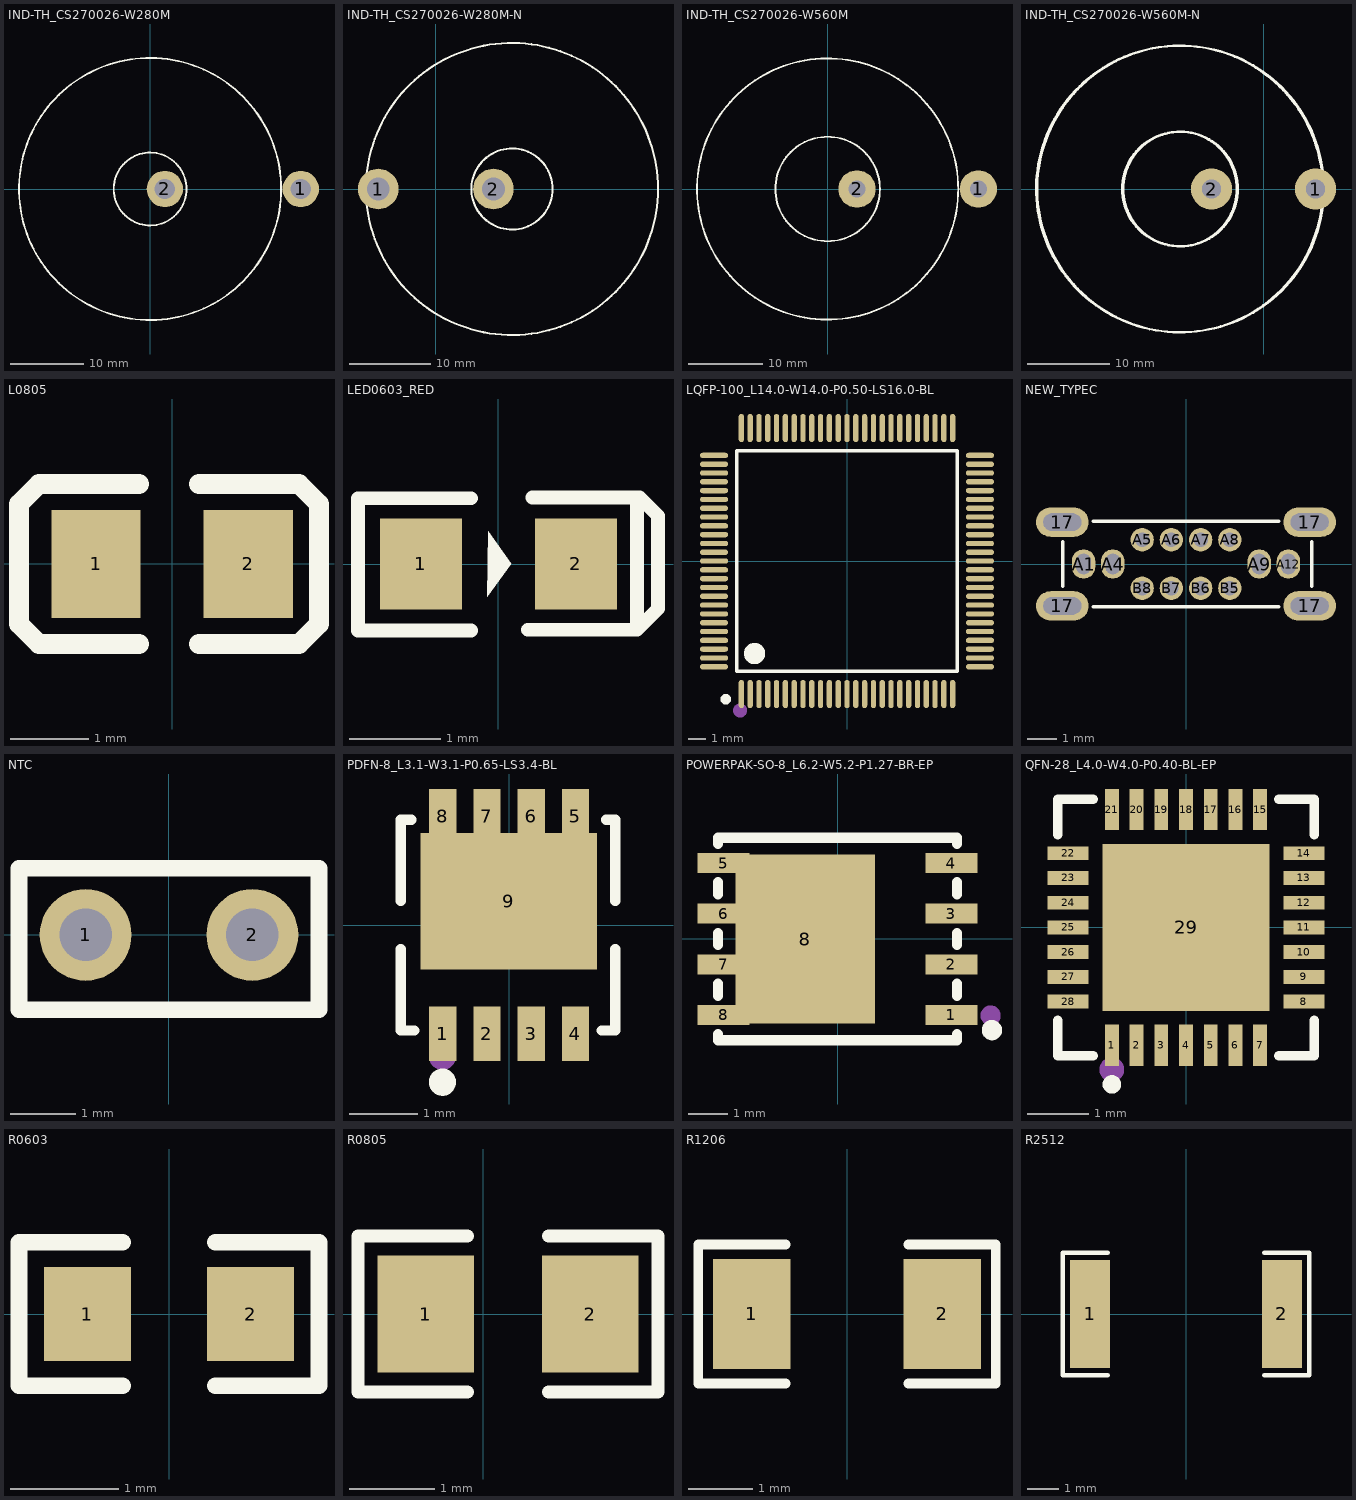
[diagram p0: the footprints below, top view; thin cyan lines are the x and y axes]
# Altium footprint library MISC84402-3.PcbLib: 74 footprints (part 3 of 5)
Each footprint in its own frame and in the unit in brackets; x right, y up, seen from the top. Pads: shape width x height; smd on the part's side, far side on the other; paste and mask are expansions set on the pad; w line width, h text height; cw(c..) or ccw(c..) is an arc to the next point about the centre after c.

## IND-TH_CS270026-W280M [mm]
pads (2):
  round 5 hole 2.8: 1(20.701,0) 2(2.032,0)
Top Overlay:
  circle w0.254: c0,0 r18
  circle w0.254: c0,0 r5

## IND-TH_CS270026-W280M-N [mm]
pads (2):
  round 5 hole 2.8: 1(-7.096,0) 2(7.096,0)
Top Overlay:
  circle w0.254: c7.096,0 r1.4
  circle w0.254: c-7.096,0 r1.4
  circle w0.254: c9.385,0.001 r18
  circle w0.254: c9.385,0 r5
  lines w0.254: 7.096,-1.4 cw(c7.096,0) 7.096,1.4 ; 7.096,-1.4 7.101,-1.4 7.096,-1.4 ; 7.096,1.4 7.101,1.4 7.096,1.4

## IND-TH_CS270026-W560M [mm]
pads (2):
  round 5 hole 2.3: 1(20.193,0) 2(3.937,0)
Top Overlay:
  circle w0.254: c0,0 r7
  circle w0.254: c0,0 r17.5

## IND-TH_CS270026-W560M-N [mm]
pads (2):
  round 5 hole 2.3 slot 2.305 at 0 deg: 1(6.35,0) 2(-6.35,0)
Top Overlay:
  circle w0.254: c6.281,0.04 r1.15
  circle w0.254: c-6.17,-0.013 r1.15
  circle w0.254: c-10.11,-0.013 r7
  circle w0.254: c-10.11,-0.013 r17.5
  circle w0.254: c-10.112,0.013 r17.5
  circle w0.254: c-10.112,0.013 r7
  lines w0.254: -10.287,-17.5 cw(c-10.284,0) -10.281,-17.5 ; -10.287,-7 cw(c-10.288,0) -10.28,-7 ; -6.175,-1.174 -6.17,-1.174 ; -6.175,-1.174 -6.17,-1.174 ; -6.175,-1.174 -6.17,-1.174 ; -6.175,-1.174 -6.17,-1.174 ; -6.175,1.149 -6.17,1.149 ; -6.175,1.149 -6.17,1.149 ; -6.175,1.149 -6.17,1.149 ; -6.175,1.149 -6.17,1.149 ; -6.175,-1.163 -6.17,-1.163 -6.175,-1.163 ; -6.175,1.137 -6.17,1.137 -6.175,1.137

## L0805 [mm]
pads (2):
  rect 1.133x1.377 smd: 1(-0.966,0) 2(0.966,0)
Top Overlay:
  lines w0.254: -0.421,-1.016 -1.691,-1.016 -1.945,-0.762 -1.945,-0.635 -1.945,0.762 -1.691,1.016 -1.564,1.016 -0.421,1.016 ; 0.341,-1.016 1.484,-1.016 1.611,-1.016 1.865,-0.762 1.865,0.635 1.865,0.762 1.611,1.016 0.341,1.016
Top Paste:
  region: 0.36,-0.22 0.36,0.22 0.745,0.688 1.433,0.688 1.533,0.588 1.533,-0.589 1.433,-0.689 0.745,-0.689
  region: -0.36,-0.22 -0.36,0.22 -0.745,0.688 -1.433,0.688 -1.533,0.588 -1.533,-0.589 -1.433,-0.689 -0.745,-0.689

## LED0603_RED [mm]
pads (2):
  rect 0.9x1 smd: 1(-0.85,0) 2(0.85,0)
Top Overlay:
  region: -0.11,0.36 -0.12,-0.36 0.14,0
  lines w0.15: -0.3,-0.73 -1.54,-0.73 -1.54,0.72 -0.3,0.72 ; 0.32,-0.72 1.52,-0.72 ; 0.37,0.73 1.52,0.73 ; 1.52,-0.72 1.72,-0.52 1.75,-0.49 1.75,0.53 1.55,0.73 1.52,0.73 ; 1.52,-0.72 1.52,0.73

## LQFP-100_L14.0-W14.0-P0.50-LS16.0-BL [mm]
pads (100):
  oval 0.3x1.6 smd: 1(-6,-7.55) 2(-5.5,-7.55) 3(-5,-7.55) 4(-4.5,-7.55) 5(-4,-7.55) 6(-3.5,-7.55) 7(-3,-7.55) 8(-2.5,-7.55) 9(-2,-7.55) 10(-1.5,-7.55) 11(-1,-7.55) 12(-0.5,-7.55) 13(0,-7.55) 14(0.5,-7.55) 15(1,-7.55) 16(1.5,-7.55) 17(2,-7.55) 18(2.5,-7.55) 19(3,-7.55) 20(3.5,-7.55) 21(4,-7.55) 22(4.5,-7.55) 23(5,-7.55) 24(5.5,-7.55) 25(6,-7.55) 51(6,7.55) 52(5.5,7.55) 53(5,7.55) 54(4.5,7.55) 55(4,7.55) 56(3.5,7.55) 57(3,7.55) 58(2.5,7.55) 59(2,7.55) 60(1.5,7.55) 61(1,7.55) 62(0.5,7.55) 63(0,7.55) 64(-0.5,7.55) 65(-1,7.55) 66(-1.5,7.55) 67(-2,7.55) 68(-2.5,7.55) 69(-3,7.55) 70(-3.5,7.55) 71(-4,7.55) 72(-4.5,7.55) 73(-5,7.55) 74(-5.5,7.55) 75(-6,7.55)
  oval 1.6x0.3 smd: 26(7.55,-6) 27(7.55,-5.5) 28(7.55,-5) 29(7.55,-4.5) 30(7.55,-4) 31(7.55,-3.5) 32(7.55,-3) 33(7.55,-2.5) 34(7.55,-2) 35(7.55,-1.5) 36(7.55,-1) 37(7.55,-0.5) 38(7.55,0) 39(7.55,0.5) 40(7.55,1) 41(7.55,1.5) 42(7.55,2) 43(7.55,2.5) 44(7.55,3) 45(7.55,3.5) 46(7.55,4) 47(7.55,4.5) 48(7.55,5) 49(7.55,5.5) 50(7.55,6) 76(-7.55,6) 77(-7.55,5.5) 78(-7.55,5) 79(-7.55,4.5) 80(-7.55,4) 81(-7.55,3.5) 82(-7.55,3) 83(-7.55,2.5) 84(-7.55,2) 85(-7.55,1.5) 86(-7.55,1) 87(-7.55,0.5) 88(-7.55,0) 89(-7.55,-0.5) 90(-7.55,-1) 91(-7.55,-1.5) 92(-7.55,-2) 93(-7.55,-2.5) 94(-7.55,-3) 95(-7.55,-3.5) 96(-7.55,-4) 97(-7.55,-4.5) 98(-7.55,-5) 99(-7.55,-5.5) 100(-7.55,-6)
Top Overlay:
  lines w0.2: -6.25,-6.25 6.25,-6.25 6.25,6.25 -6.25,6.25 -6.25,-6.25
  lines w0.3: -6.883,-7.696 ccw(c-6.882,-7.846) -6.881,-7.696
  lines w0.6: -5.25,-4.95 ccw(c-5.248,-5.25) -5.245,-4.95
Mechanical 15:
  circle w0.4: c-6.071,-8.484 r0.2

## NEW_TYPEC [mm]
pads (16):
  oval 1.8x1 hole 0.6 slot 1.3 at 0 deg: 17(-4.225,-1.43) 17(-4.225,1.43) 17(4.225,-1.43) 17(4.225,1.43)
  oval 0.8x1 hole 0.5 slot 0.7 at 90 deg: A1(-3.5,0) A4(-2.5,0) A9(2.5,0) A12(3.5,0)
  round 0.8 hole 0.5: A5(-1.5,0.825) A6(-0.5,0.825) A7(0.5,0.825) A8(1.5,0.825) B5(1.5,-0.825) B6(0.5,-0.825) B7(-0.5,-0.825) B8(-1.5,-0.825)
Top Overlay:
  lines w0.127: -4.215,-0.762 -4.215,0.762 ; -3.158,-1.46 3.158,-1.46 ; -3.158,1.461 3.158,1.461 ; 4.294,-0.762 4.294,0.762

## NTC [mm]
pads (2):
  round 1.4 hole 0.8: 1(-1.27,0) 2(1.27,0)
Top Overlay:
  lines w0.254: -2.286,-1.143 2.286,-1.143 2.286,1.016 -2.286,1.016 -2.286,-1.143

## PDFN-8_L3.1-W3.1-P0.65-LS3.4-BL [mm]
pads (9):
  rect 0.4x0.8 smd: 1(-0.975,-1.6) 2(-0.325,-1.6) 3(0.325,-1.6) 4(0.975,-1.6) 5(0.975,1.6) 6(0.325,1.6) 7(-0.325,1.6) 8(-0.975,1.6)
  rect 2.6x2 smd: 9(-0.005,0.35)
Top Overlay:
  circle w0.2: c-0.98,-2.31 r0.1
  lines w0.152: -1.592,-0.354 -1.592,-1.55 -1.396,-1.55 ; -1.592,0.354 -1.592,1.55 -1.434,1.55 ; 1.362,-1.55 1.56,-1.55 1.56,-0.354 ; 1.425,1.55 1.56,1.55 1.56,0.354
Top Paste:
  region: 1.175,1.5 0.775,1.5 0.775,2 1.175,2
  region: 0.525,1.5 0.125,1.5 0.125,2 0.525,2
  region: -0.125,1.5 -0.525,1.5 -0.525,2 -0.125,2
  region: -1.31,1.22 1.293,1.22 1.293,-0.649 -1.307,-0.649
  region: -1.175,-2 -1.175,-1.2 -0.775,-1.2 -0.775,-2
  region: -0.525,-2 -0.525,-1.2 -0.125,-1.2 -0.125,-2
  region: 0.125,-2 0.125,-1.2 0.525,-1.2 0.525,-2
  region: 0.775,-2 0.775,-1.2 1.175,-1.2 1.175,-2
  region: -0.775,1.5 -1.175,1.5 -1.175,2 -0.775,2
Mechanical 15:
  circle w0.2: c-0.98,-1.93 r0.1

## POWERPAK-SO-8_L6.2-W5.2-P1.27-BR-EP [mm]
pads (9):
  rect 1.3x0.5 smd: 1(2.858,-1.905) 2(2.858,-0.635) 3(2.858,0.635) 4(2.858,1.905) 5(-2.858,1.905) 6(-2.858,0.635) 7(-2.858,-0.635) 8(-2.858,-1.905)
  rect 3.5x4.25 smd: 8(-0.813,0)
Top Overlay:
  circle w0.254: c3.873,-2.286 r0.127
  lines w0.254: -3,-2.386 -3,-2.54 3,-2.54 3,-2.386 ; -3,-1.424 -3,-1.116 ; -3,-0.154 -3,0.154 ; -3,1.116 -3,1.424 ; -3,2.386 -3,2.54 3,2.54 3,2.386 ; 3,-1.424 3,-1.116 ; 3,-0.154 3,0.154 ; 3,1.116 3,1.424
Top Paste:
  region: -3.525,1.625 -3.525,2.145 -2.225,2.145 -2.225,1.625
  region: -3.525,0.355 -3.525,0.875 -2.225,0.875 -2.225,0.355
  region: -3.525,-0.915 -3.525,-0.395 -2.225,-0.395 -2.225,-0.915
  region: -3.525,-2.185 -3.525,-1.665 -2.225,-1.665 -2.225,-2.185
  region: 2.19,1.625 2.19,2.145 3.49,2.145 3.49,1.625
  region: 2.19,0.355 2.19,0.875 3.49,0.875 3.49,0.355
  region: 2.19,-0.915 2.19,-0.395 3.49,-0.395 3.49,-0.915
  region: 2.19,-2.185 2.19,-1.665 3.49,-1.665 3.49,-2.185
  region: -1.94,-1.978 -1.94,-0.158 0.86,-0.158 0.86,-1.978
  region: 0.86,1.991 0.86,0.171 -1.94,0.171 -1.94,1.991
Mechanical 15:
  circle w0.254: c3.84,-1.92 r0.127

## QFN-28_L4.0-W4.0-P0.40-BL-EP [mm]
pads (29):
  rect 0.224x0.665 smd: 1(-1.2,-1.907) 2(-0.8,-1.907) 3(-0.4,-1.907) 4(0,-1.907) 5(0.4,-1.907) 6(0.8,-1.907) 7(1.2,-1.907) 15(1.2,1.908) 16(0.8,1.908) 17(0.4,1.908) 18(0,1.908) 19(-0.4,1.908) 20(-0.8,1.908) 21(-1.2,1.908)
  rect 0.665x0.224 smd: 8(1.907,-1.2) 9(1.907,-0.8) 10(1.907,-0.4) 11(1.907,0) 12(1.907,0.4) 13(1.907,0.8) 14(1.907,1.2) 22(-1.907,1.2) 23(-1.907,0.8) 24(-1.907,0.4) 25(-1.907,0) 26(-1.907,-0.4) 27(-1.907,-0.8) 28(-1.907,-1.2)
  rect 2.7x2.7 smd: 29(0,0)
Top Overlay:
  circle w0.15: c-1.2,-2.54 r0.075
  lines w0.152: -2.076,-1.503 -2.076,-2.076 -1.503,-2.076 ; -2.076,1.503 -2.076,2.076 -1.503,2.076 ; 1.503,-2.076 2.076,-2.076 2.076,-1.503 ; 1.503,2.076 2.076,2.076 2.076,1.503
Mechanical 15:
  circle w0.2: c-1.2,-2.3 r0.1

## R0603 [mm]
pads (2):
  rect 0.806x0.864 smd: 1(-0.753,0) 2(0.753,0)
Top Overlay:
  lines w0.152: -0.426,-0.661 -1.385,-0.661 -1.385,0.661 -0.426,0.661 ; 0.426,-0.661 1.385,-0.661 1.385,0.661 0.426,0.661
Top Paste:
  region: 1.195,0.45 0.395,0.45 0.345,0.4 0.345,0.172 0.715,0.172 0.715,-0.158 0.345,-0.158 0.345,-0.4 0.395,-0.45 1.195,-0.45 1.245,-0.4 1.245,0.4
  region: -0.355,0.4 -0.355,0.172 -0.735,0.172 -0.735,-0.158 -0.355,-0.158 -0.355,-0.4 -0.405,-0.45 -1.195,-0.45 -1.245,-0.4 -1.245,0.4 -1.195,0.45 -0.405,0.45

## R0805 [mm]
pads (2):
  rect 1.133x1.377 smd: 1(-0.678,0) 2(1.254,0)
Top Overlay:
  lines w0.152: -0.188,-0.917 -1.473,-0.917 -1.473,0.917 -0.188,0.917 ; 0.764,-0.917 2.049,-0.917 2.049,0.917 0.764,0.917
Top Paste:
  region: 0.738,-0.64 0.738,-0.22 1.183,-0.22 1.183,0.23 0.743,0.23 0.738,0.64 0.788,0.69 1.938,0.69 1.988,0.64 1.988,-0.64 1.938,-0.69 0.788,-0.69
  region: -1.412,-0.64 -1.412,0.64 -1.362,0.69 -0.212,0.69 -0.162,0.64 -0.157,0.23 -0.607,0.23 -0.607,-0.22 -0.167,-0.22 -0.162,-0.64 -0.212,-0.69 -1.362,-0.69

## R1206 [mm]
height 12.5
pads (2):
  rect 1.208x1.701 smd: 1(-1.479,0) 2(1.479,0)
Top Overlay:
  lines w0.152: -0.951,-1.079 -2.311,-1.079 -2.311,1.079 -0.951,1.079 ; 0.951,-1.079 2.311,-1.079 2.311,1.079 0.951,1.079
Top Paste:
  region: 0.875,-0.75 0.875,-0.389 0.975,-0.289 1.186,-0.289 1.286,-0.189 1.286,0.189 1.186,0.289 0.975,0.289 0.875,0.389 0.875,0.75 0.975,0.85 1.983,0.85 2.083,0.75 2.083,-0.75 1.983,-0.85 0.975,-0.85
  region: -0.875,-0.75 -0.875,-0.389 -0.975,-0.289 -1.186,-0.289 -1.286,-0.189 -1.286,0.189 -1.186,0.289 -0.975,0.289 -0.875,0.389 -0.875,0.75 -0.975,0.85 -1.983,0.85 -2.083,0.75 -2.083,-0.75 -1.983,-0.85 -0.975,-0.85

## R2512 [mm]
pads (2):
  rect 1.283x3.456 smd: 1(-3.066,0) 2(3.066,0)
Top Overlay:
  lines w0.152: -2.501,-1.957 -3.936,-1.957 -3.936,1.957 -2.501,1.957 ; 2.501,-1.957 3.936,-1.957 3.936,1.957 2.501,1.957
Top Paste:
  region: 2.425,-1.628 2.425,-0.688 2.525,-0.588 2.761,-0.588 2.861,-0.488 2.861,0.488 2.761,0.588 2.525,0.588 2.425,0.688 2.425,1.628 2.525,1.728 3.608,1.728 3.708,1.628 3.708,-1.628 3.608,-1.728 2.525,-1.728
  region: -2.425,-1.628 -2.425,-0.688 -2.525,-0.588 -2.761,-0.588 -2.861,-0.488 -2.861,0.488 -2.761,0.588 -2.525,0.588 -2.425,0.688 -2.425,1.628 -2.525,1.728 -3.608,1.728 -3.708,1.628 -3.708,-1.628 -3.608,-1.728 -2.525,-1.728